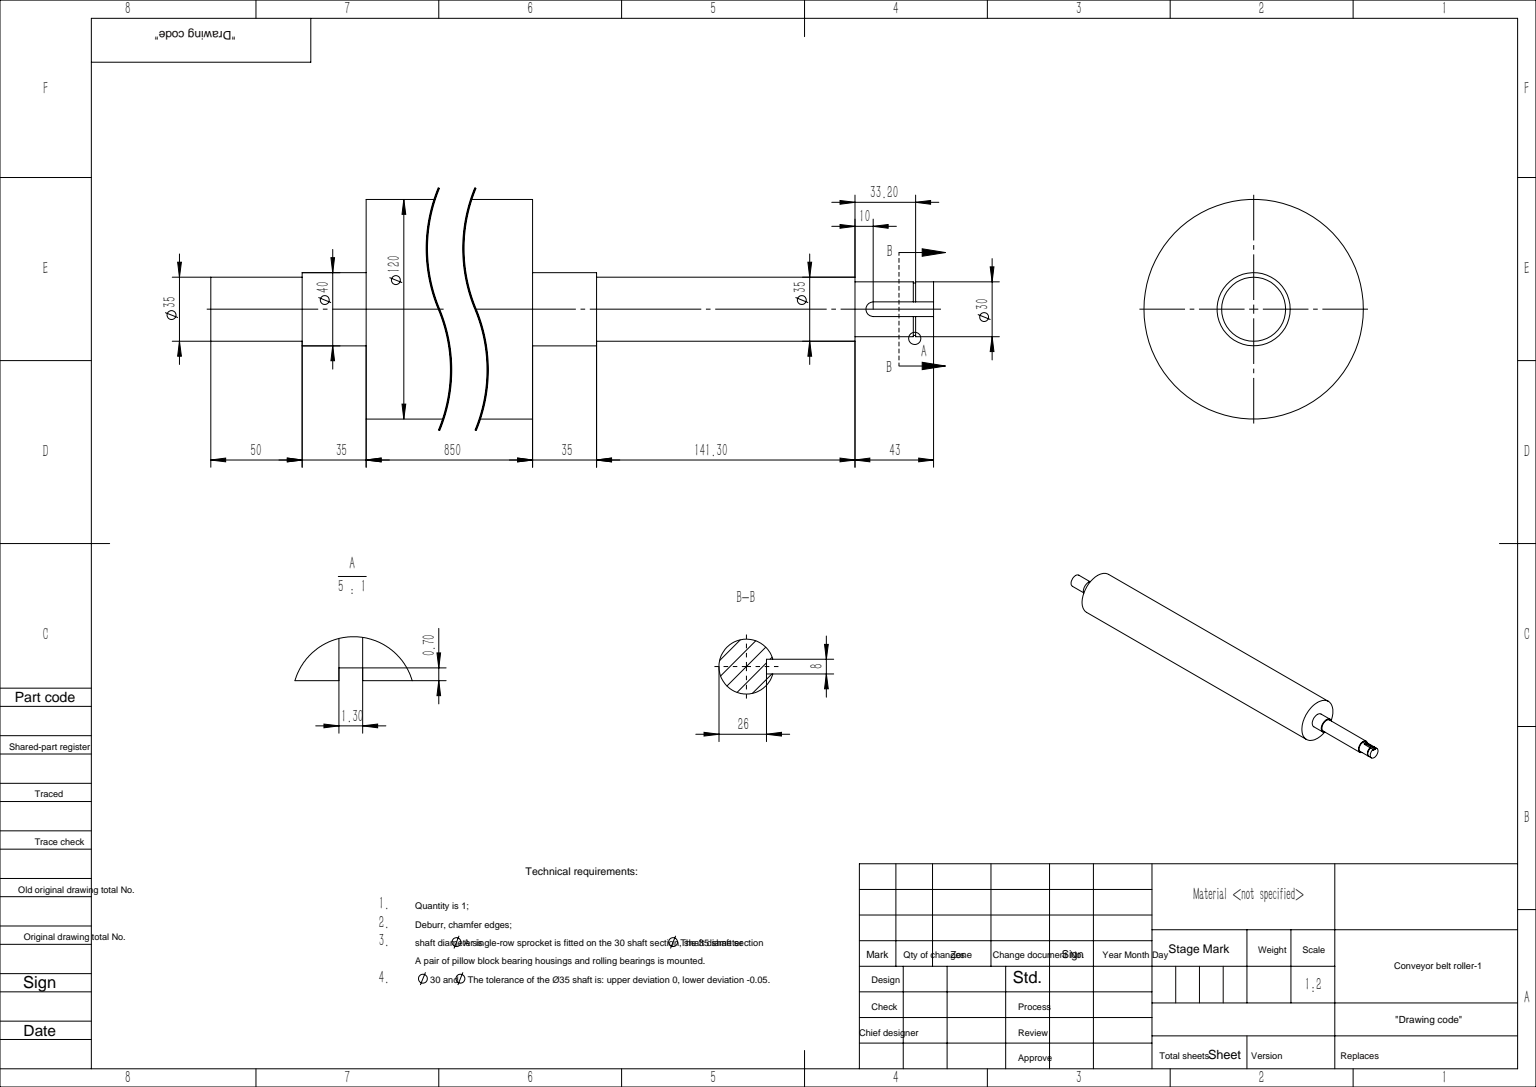
from build123d import *

# Parameters (mm, degrees)
CUT_EXTRUDE_1_DEPTH = 4
SKETCH_3_R          = 15
SKETCH_3_R_2        = 14.3
CUT_EXTRUDE_3_DEPTH = 1.3


with BuildPart() as part:
    # 草图1 → 旋转1 (revolve)
    with BuildSketch(Plane.XY):
        Polygon((0, 0), (0, 17.5), (50, 17.5), (50, 20), (85, 20), (85, 60), (935, 60), (935, 20), (970, 20), (970, 17.5), (1111.3, 17.5), (1111.3, 15), (1154.3, 15), (1154.3, 0), align=None)
    revolve(axis=Axis((1154.3, 0, 0), (-1, 0, 0)))

    # 草图2 → 切除-拉伸1 (cut)
    with BuildSketch(Plane(origin=(0, 15, 0), x_dir=(1, 0, 0), z_dir=(0, 1, 0))):
        with BuildLine():
            Line((1121.3, 4), (1164.3, 4))
            Line((1164.3, 4), (1164.3, -4))
            Line((1164.3, -4), (1121.3, -4))
            ThreePointArc((1121.3, -4), (1117.3, 0), (1121.3, 4))
        make_face()
    extrude(amount=-CUT_EXTRUDE_1_DEPTH, mode=Mode.SUBTRACT)

    # 草图3 → 切除-拉伸3 (cut)
    with BuildSketch(Plane(origin=(1144.5, 0, 0), x_dir=(0, 0, -1), z_dir=(1, 0, 0))):
        with Locations(Location((0, 0, 0), (0, 0, 90))):
            Circle(SKETCH_3_R)
        Circle(SKETCH_3_R_2, mode=Mode.SUBTRACT)
    extrude(amount=-CUT_EXTRUDE_3_DEPTH, mode=Mode.SUBTRACT)


solid = part.part
